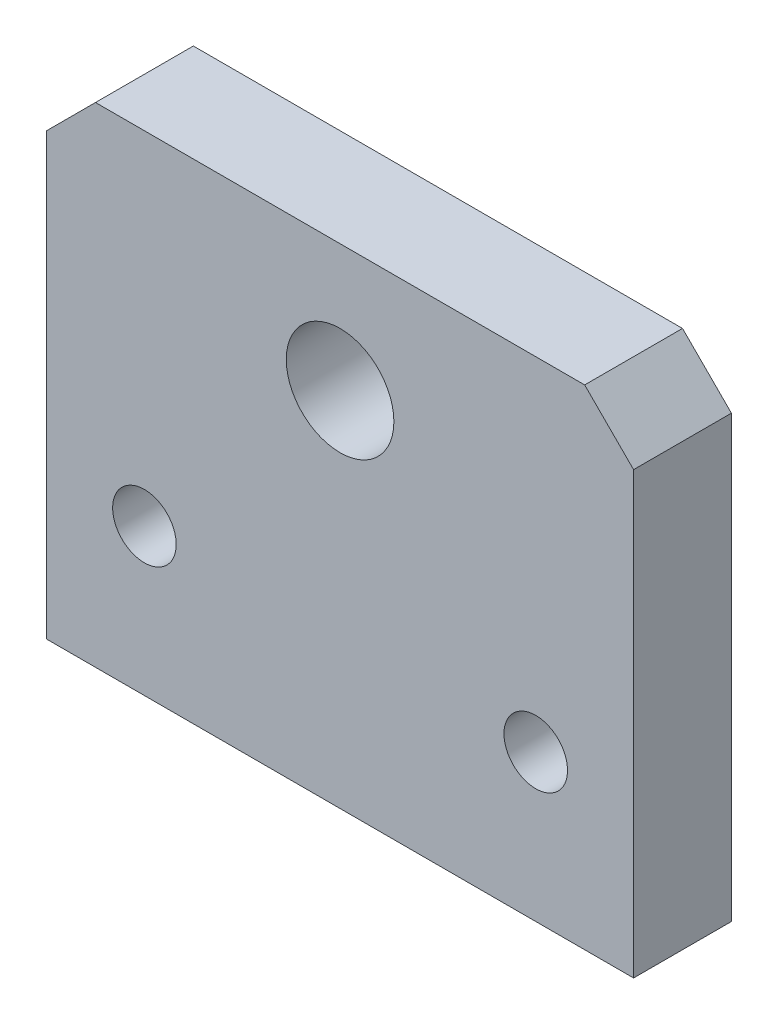
SolidWorks part; units mm, degrees
ref_plane "Front Plane" through (0, 0, 0) normal (0, 0, 1) x (1, 0, 0)
ref_plane "Top Plane" through (0, 0, 0) normal (0, 1, 0) x (1, 0, 0)
ref_plane "Right Plane" through (0, 0, 0) normal (1, 0, 0) x (0, 0, -1)
sketch "Sketch1" plane through (0, 0, 0) normal (0, 0, 1) x (1, 0, 0)
  line L1 (-35.2439, 22.2348) -> (24.7561, 22.2348)
  line L2 (-35.2439, 22.2348) -> (-35.2439, -27.7652)
  line L3 (-35.2439, -27.7652) -> (24.7561, -27.7652)
  line L4 (24.7561, 22.2348) -> (24.7561, -27.7652)
  dimension "D1" = 60
  dimension "D2" = 50
extrude "Boss-Extrude1" add sketch "Sketch1" along normal blind 10
sketch "Sketch2" plane through (0, 0, 0) normal (0, 0, -1) x (-1, 0, 0)
  circle A0 centre (5.2439, 9.2348) radius 5.5
  dimension "D1" = 11
extrude "Cut-Extrude1" cut sketch "Sketch2" against normal blind 18
chamfer "Chamfer1" distance 5 angle 45 2 edges at (-35.2439, 22.2348, 5) (24.7561, 22.2348, 5)
sketch "Sketch3" plane through (0, 0, 0) normal (0, 0, -1) x (-1, 0, 0)
  circle A0 centre (-14.7561, -12.7652) radius 3.25
  circle A1 centre (25.2439, -12.7652) radius 3.25
  dimension "D1" = 6.5
extrude "Cut-Extrude2" cut sketch "Sketch3" against normal through all
